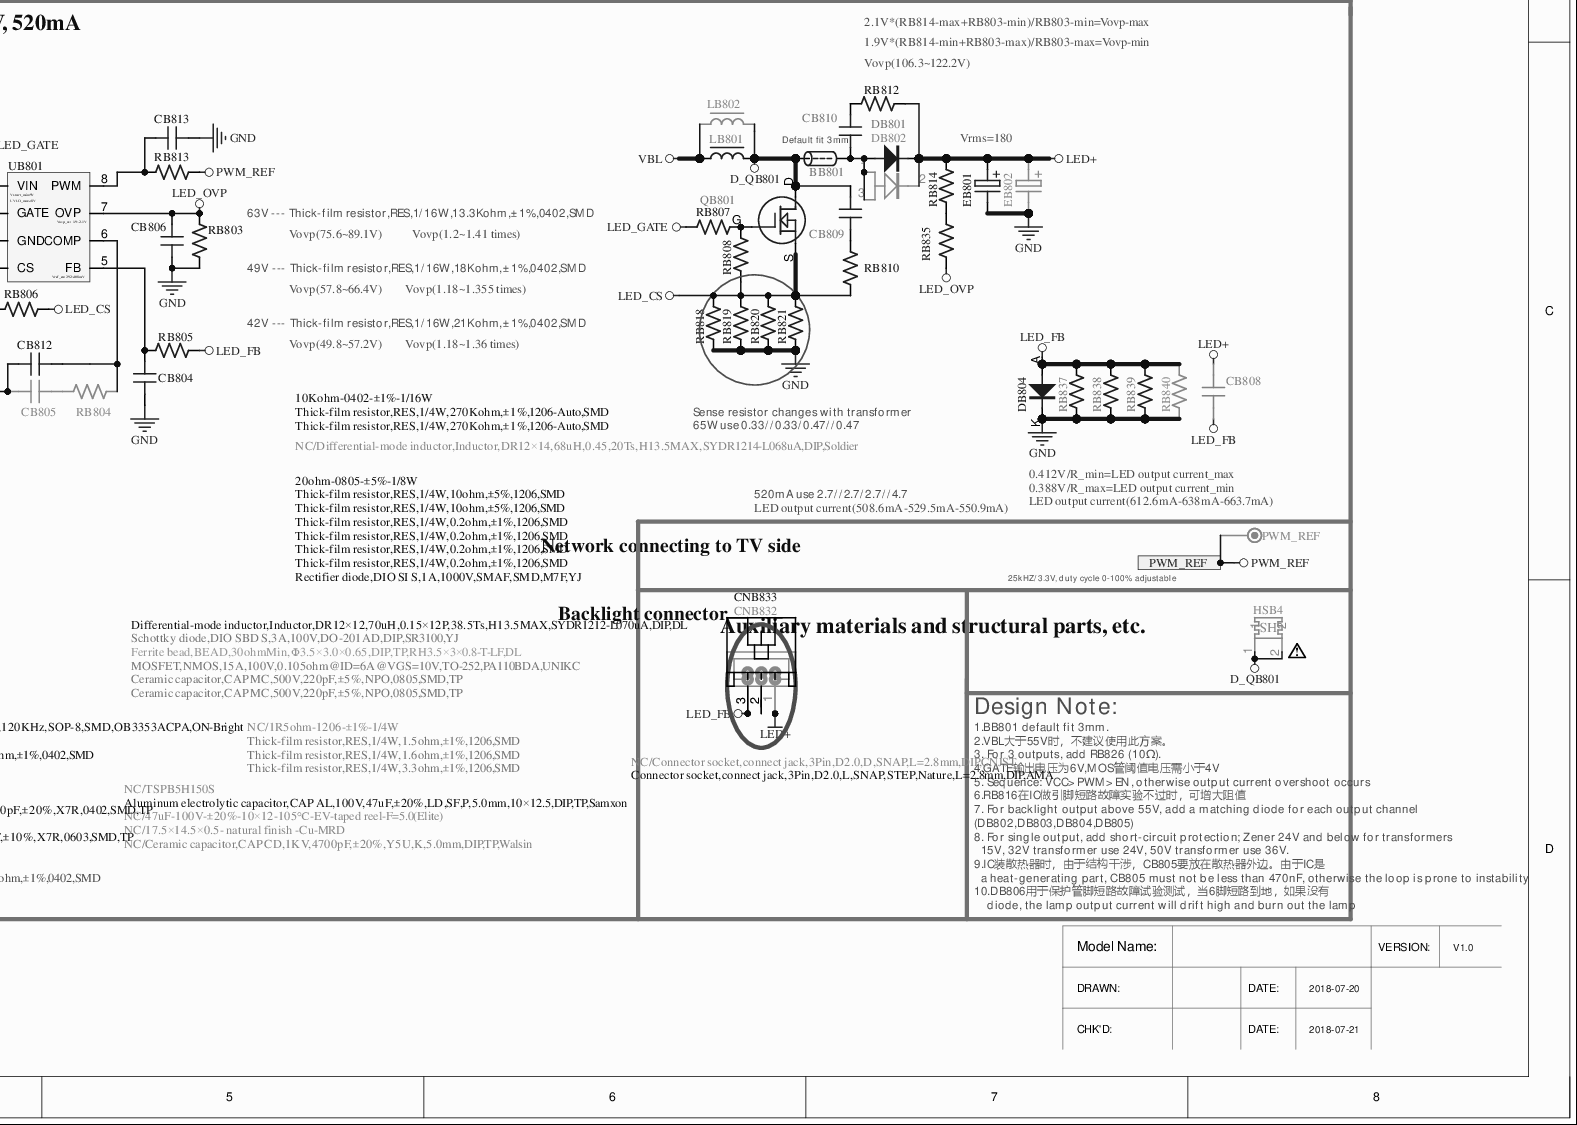
[diagram p0: MISC84438-4.SchDoc, bottom right]
# Altium project MISC84438-18.PrjPCB (part 8 of 8)

## Nets that join several sheets
1.15V_STB: MISC84438-7 (7 pins), MISC84438-8 (14 pins)
3V3_STB: MISC84438-7 (7 pins), MISC84438-8 (25 pins), MISC84438-9 (RF20.2 RF26.1 RK4.2 RK18.2)
3V3_TU: MISC84438-7 (7 pins), MISC84438-13 (CT3.1 LT12.1)
5V_M: MISC84438-7 (8 pins), MISC84438-10 (F1.2 F2.1 RO2.2 RO6.1)
5V_STB: MISC84438-7 (18 pins), MISC84438-9 (RK1.2 RK13.1 RK15.1), MISC84438-11 (RF8.2 RF9.2)
12V: MISC84438-7 (6 pins), MISC84438-12 (12 pins), MISC84438-4 (14 pins)
+1.8V_DDR: MISC84438-7 (7 pins), MISC84438-8 (7 pins)
GND: MISC84438-3 (36 pins), MISC84438-7 (44 pins), MISC84438-8 (37 pins), MISC84438-9 (43 pins), MISC84438-10 (60 pins), MISC84438-11 (20 pins), MISC84438-12 (25 pins), MISC84438-13 (45 pins), MISC84438-4 (39 pins)
PWM_REF: MISC84438-7 (CG1.1 RG1.2 RG1.3), MISC84438-4 (PWM_REF.1 RB813.2)
VCC_PANEL: MISC84438-7 (5 pins), MISC84438-9 (9 pins)
AMP-OUTL: MISC84438-8 (CF29.1 RF14.2 U1.41), MISC84438-12 (RA21.1)
AMP-OUTR: MISC84438-8 (CF30.1 RF15.2 U1.42), MISC84438-12 (RA5.1)
AMP_STB: MISC84438-8 (U1.81), MISC84438-12 (RA1.2 RA8.1)
AV1_LIN: MISC84438-8 (U1.32), MISC84438-10 (CI7.1)
AV1_RIN: MISC84438-8 (U1.31), MISC84438-10 (CI6.1)
AV2_LIN: MISC84438-8 (U1.36), MISC84438-10 (CI4.1)
AV2_RIN: MISC84438-8 (U1.35), MISC84438-10 (CI3.1)
AV-OUTL: MISC84438-8 (U1.39), MISC84438-10 (CO3.2 RO1.1 RO4.2)
AV-OUTR: MISC84438-8 (U1.40), MISC84438-10 (CO5.2 RO5.1 RO8.2)
AV_IN: MISC84438-8 (U1.27), MISC84438-10 (CI8.1)
CVBS_OUT: MISC84438-8 (U1.29), MISC84438-10 (CO9.2 RO12.1 RO14.2)
DDC_SCL/UART_RX: MISC84438-10 (AVV1.15 DV2.K), MISC84438-11 (CN9.2 RF8.1 RF11.1 RH2.2)
DDC_SDA/UART_TX: MISC84438-10 (AVV1.12 DV1.K), MISC84438-11 (CN9.3 RF9.1 RF10.1 RH1.2)
EXE_IR: MISC84438-8 (U1.80), MISC84438-10 (RO6.2 RO9.2 RO10.2)
GIN0N: MISC84438-8 (U1.19), MISC84438-10 (CF31.1)
GIN1N: MISC84438-8 (U1.25), MISC84438-10 (CF34.2)
HDMI1_HPDIN: MISC84438-8 (U1.113), MISC84438-11 (RPH2.6 RPH2.8)
HDMI1_RX0_N: MISC84438-8 (U1.1), MISC84438-11 (AVH1.9)
HDMI1_RX0_P: MISC84438-8 (U1.2), MISC84438-11 (AVH1.7)
HDMI1_RX1_N: MISC84438-8 (U1.3), MISC84438-11 (AVH1.6)
HDMI1_RX1_P: MISC84438-8 (U1.4), MISC84438-11 (AVH1.4)
HDMI1_RX2_N: MISC84438-8 (U1.5), MISC84438-11 (AVH1.3)
HDMI1_RX2_P: MISC84438-8 (U1.6), MISC84438-11 (AVH1.1)
HDMI1_RXC_N: MISC84438-8 (U1.127), MISC84438-11 (AVH1.12)
HDMI1_RXC_P: MISC84438-8 (U1.128), MISC84438-11 (AVH1.10)
HDMI1_SCL: MISC84438-8 (U1.108), MISC84438-11 (RH10.1)
HDMI1_SDA: MISC84438-8 (U1.107), MISC84438-11 (RH11.1)
HDMI_ARC: MISC84438-8 (U1.117), MISC84438-11 (CH15.2)
HDMI_CEC: MISC84438-8 (U1.111), MISC84438-11 (RH13.2)
HDMI_DET: MISC84438-8 (U1.102), MISC84438-11 (RH28.1 RH29.1)
IFAGC: MISC84438-8 (U1.43), MISC84438-13 (CT19.2 RT2.2 RT18.2)
KEY1: MISC84438-8 (U1.101), MISC84438-9 (CK2.1 RK3.1)
LED_RED: MISC84438-8 (U1.83), MISC84438-9 (RK18.1 RK20.2 RK21.1)
M_SCL: MISC84438-8 (RT3.2 U1.52), MISC84438-9 (RF23.1 RF25.1), MISC84438-13 (DT3.K RT6.1)
M_SDA: MISC84438-8 (RT4.2 U1.51), MISC84438-9 (RF27.1), MISC84438-13 (DT2.K RT5.1)
PANEL_ON/OFF: MISC84438-7 (RM8.1 RM10.1), MISC84438-8 (U1.82)
PWM1: MISC84438-7 (RG1.1), MISC84438-8 (R2.1 U1.87)
PWR_ON/OFF: MISC84438-7 (RM3.2 RM4.2), MISC84438-8 (U1.84)
REMOTE: MISC84438-8 (U1.88), MISC84438-9 (CK6.2 RK16.1)
RXE0+: MISC84438-8 (U1.69), MISC84438-9 (CNF1.18 CNF2.18 E0P.1)
RXE0-: MISC84438-8 (U1.70), MISC84438-9 (CNF1.19 CNF2.19 E0N.1)
RXE1+: MISC84438-8 (U1.67), MISC84438-9 (CNF1.15 CNF2.15 E1P.1)
RXE1-: MISC84438-8 (U1.68), MISC84438-9 (CNF1.16 CNF2.16 E1N.1)
RXE2+: MISC84438-8 (U1.65), MISC84438-9 (CNF1.12 CNF2.12 E2P.1)
RXE2-: MISC84438-8 (U1.66), MISC84438-9 (CNF1.13 CNF2.13 E2N.1)
RXE3+: MISC84438-8 (U1.61), MISC84438-9 (CNF1.6 CNF2.6 E3P.1)
RXE3-: MISC84438-8 (U1.62), MISC84438-9 (CNF1.7 CNF2.7 E3N.1)
RXEC+: MISC84438-8 (U1.63), MISC84438-9 (CF35.2 CNF1.9 CNF2.9 ECP.1)
RXEC-: MISC84438-8 (U1.64), MISC84438-9 (CF33.2 CNF1.10 CNF2.10 ECN.1)
UART_RX: MISC84438-8 (U1.96), MISC84438-11 (DH9.K RF11.2)
UART_TX: MISC84438-8 (U1.95), MISC84438-11 (DH8.K RF10.2)
USB0_DM: MISC84438-8 (U1.59), MISC84438-10 (DU2.K RU2.2 RU2.3)
USB0_DP: MISC84438-8 (U1.60), MISC84438-10 (DU1.K RU4.2 RU4.3)
VGA_BIN: MISC84438-8 (U1.17), MISC84438-10 (CV7.1)
VGA_GIN: MISC84438-8 (U1.18), MISC84438-10 (CV3.1)
VGA_HS: MISC84438-8 (U1.16), MISC84438-10 (CV9.2 RV12.2)
VGA_RIN: MISC84438-8 (U1.20), MISC84438-10 (CV1.1)
VGA_VS: MISC84438-8 (U1.21), MISC84438-10 (CV10.2 RV10.2)
VIFM: MISC84438-8 (U1.45), MISC84438-13 (CT23.2)
VIFP: MISC84438-8 (U1.44), MISC84438-13 (CT20.2)
XTAL_O: MISC84438-8 (CF40.1), MISC84438-13 (CT14.2 UT1.13 YT1.1)
YPBPR_Y: MISC84438-8 (U1.24), MISC84438-10 (CI1.1)